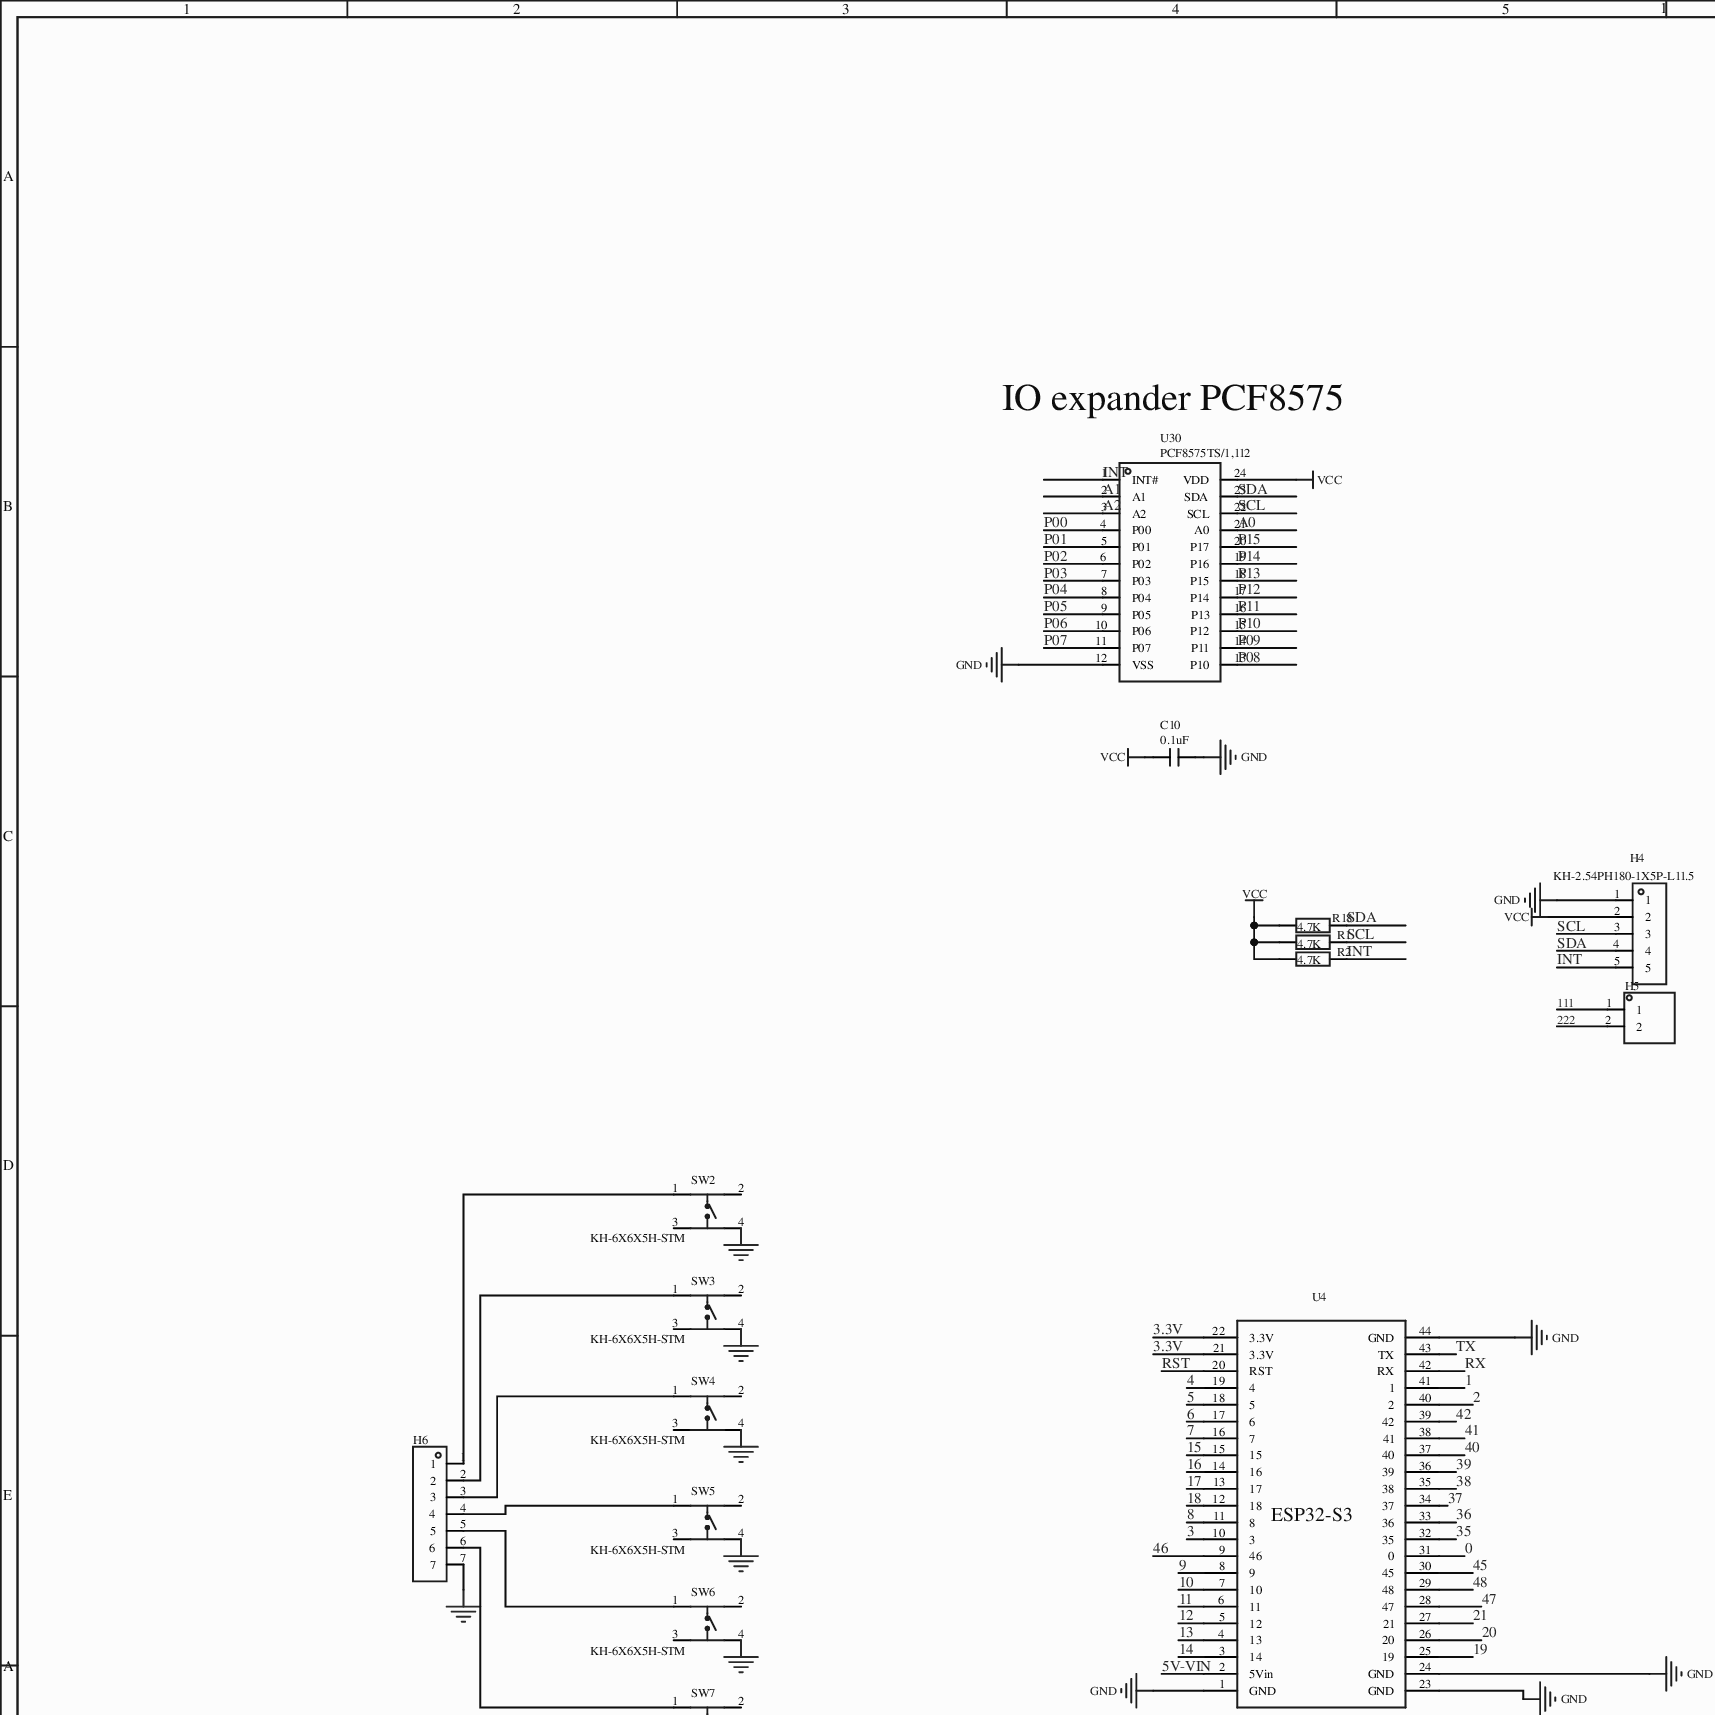
[diagram p0: MISC49879-3.schdoc, top left]
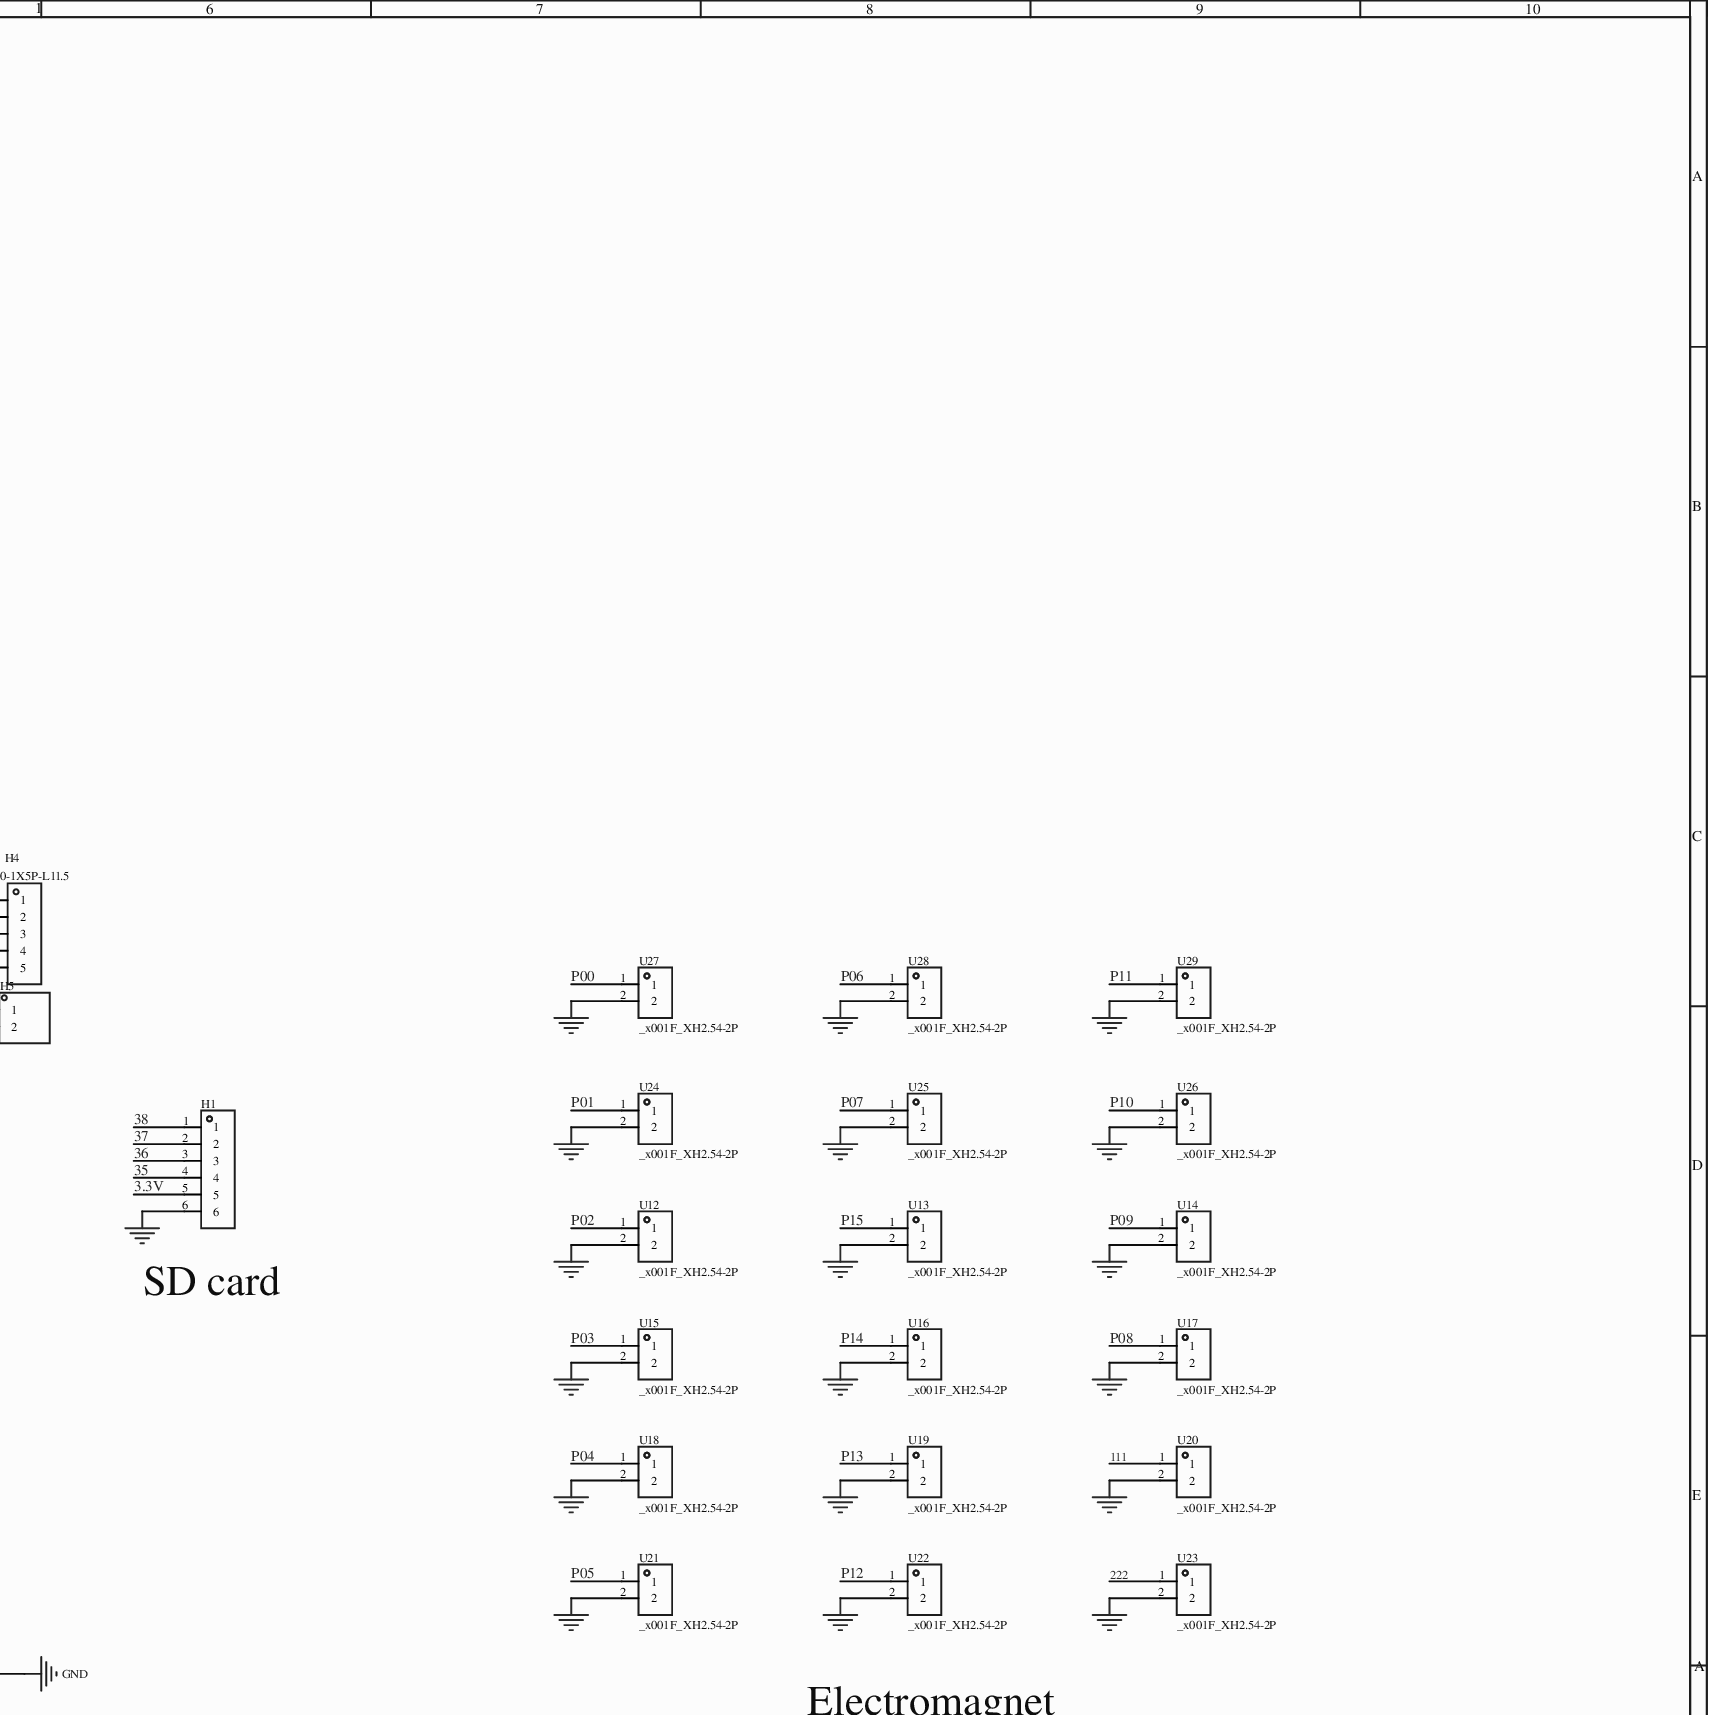
[diagram p1: MISC49879-3.schdoc, top right]
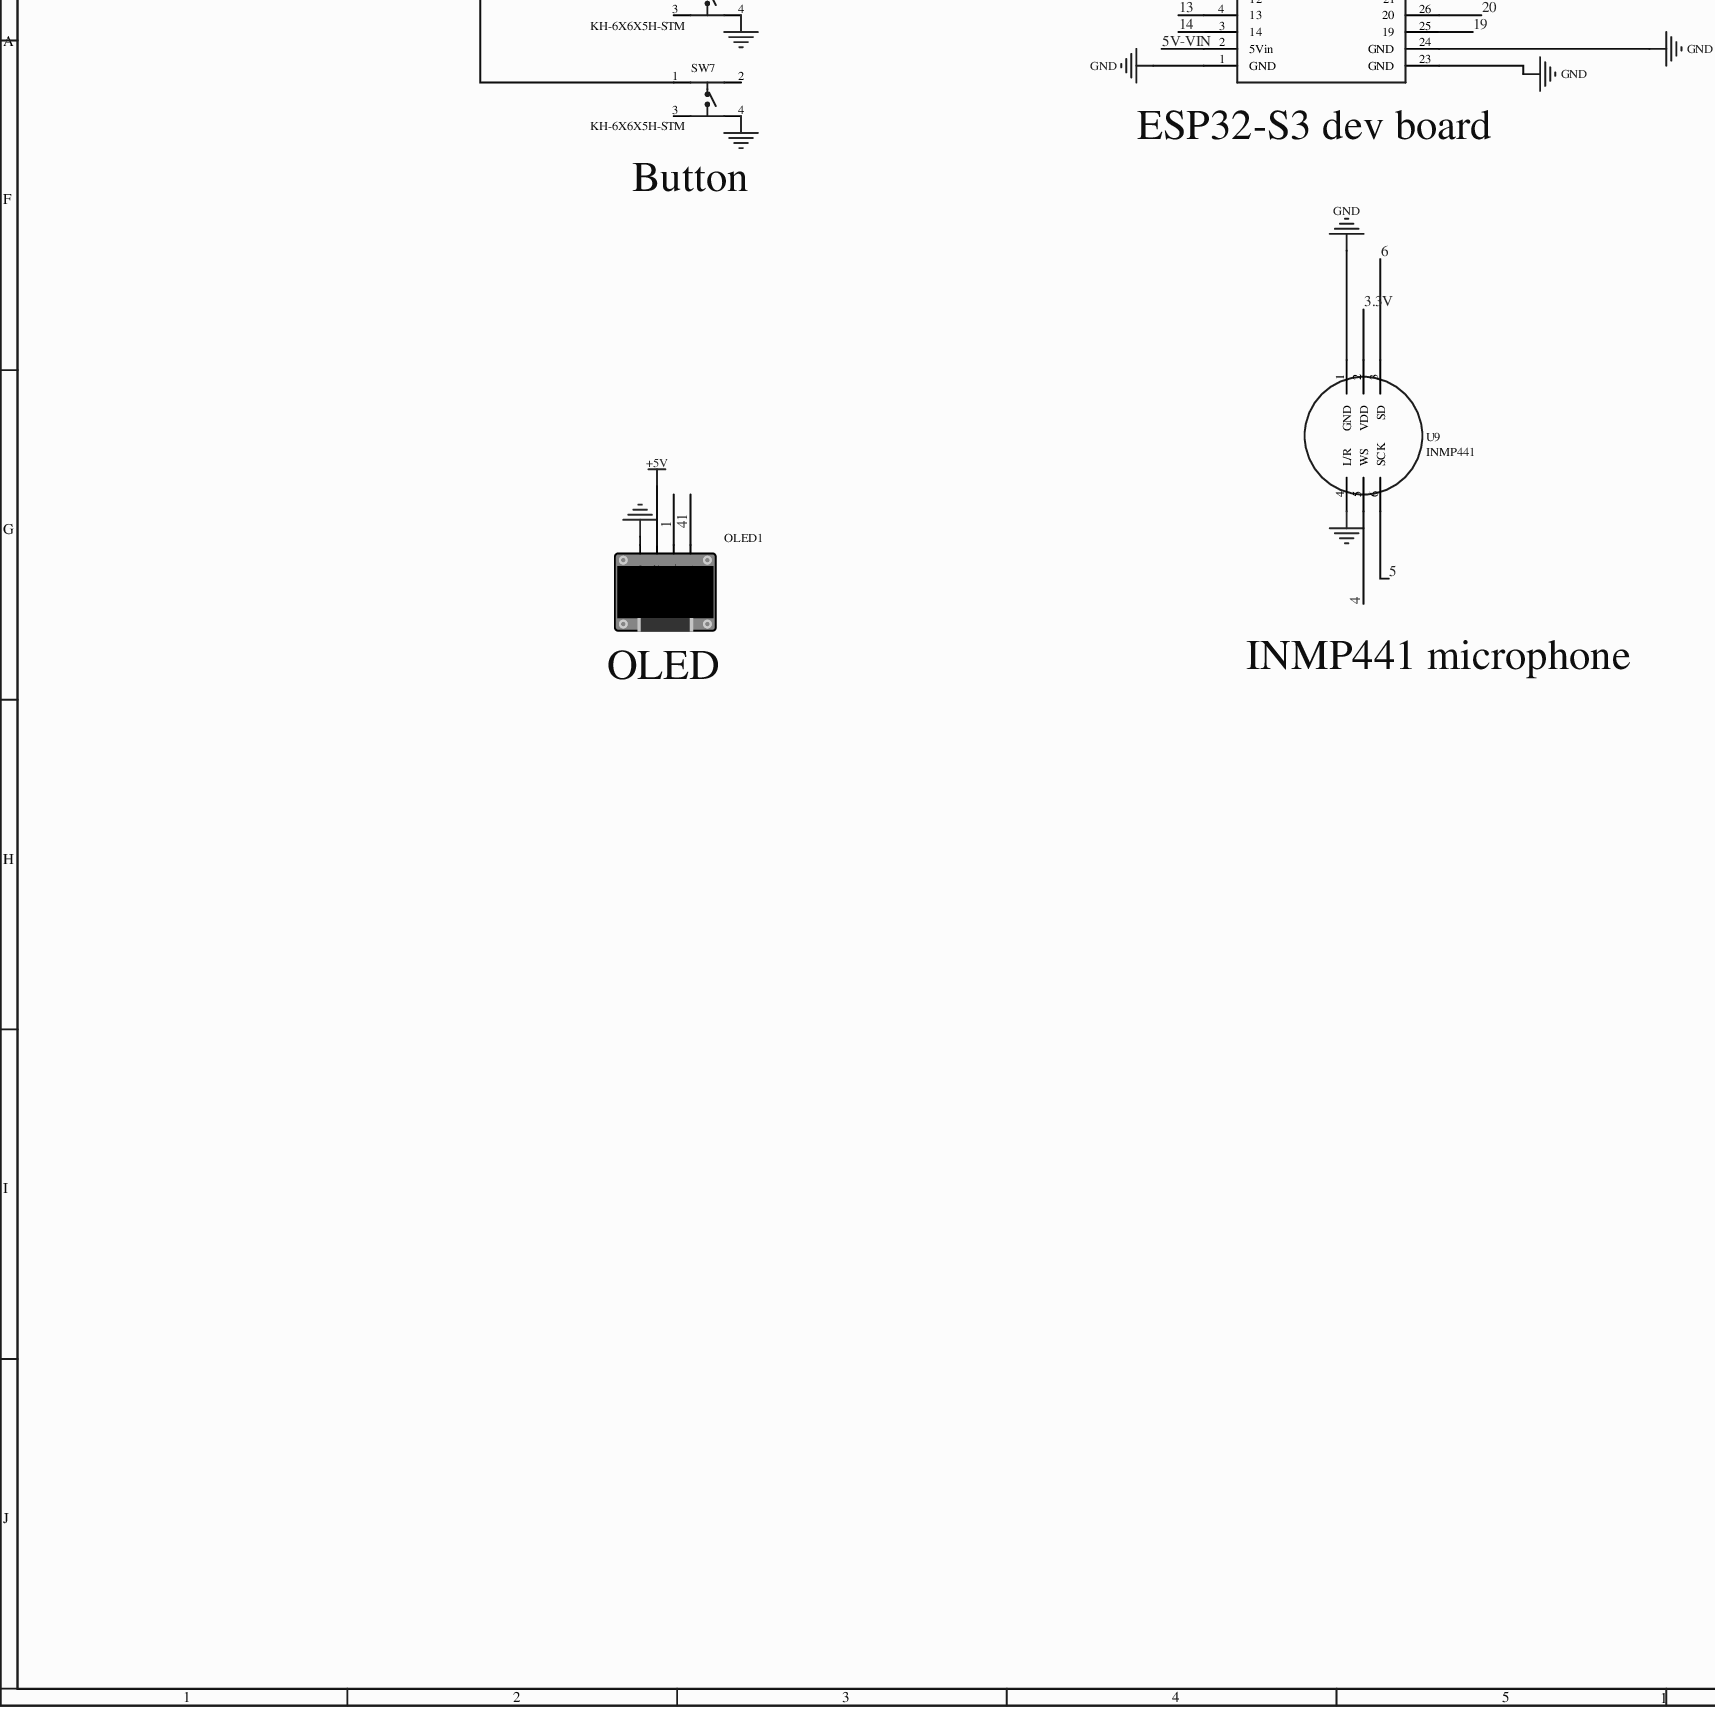
[diagram p2: MISC49879-3.schdoc, bottom left]
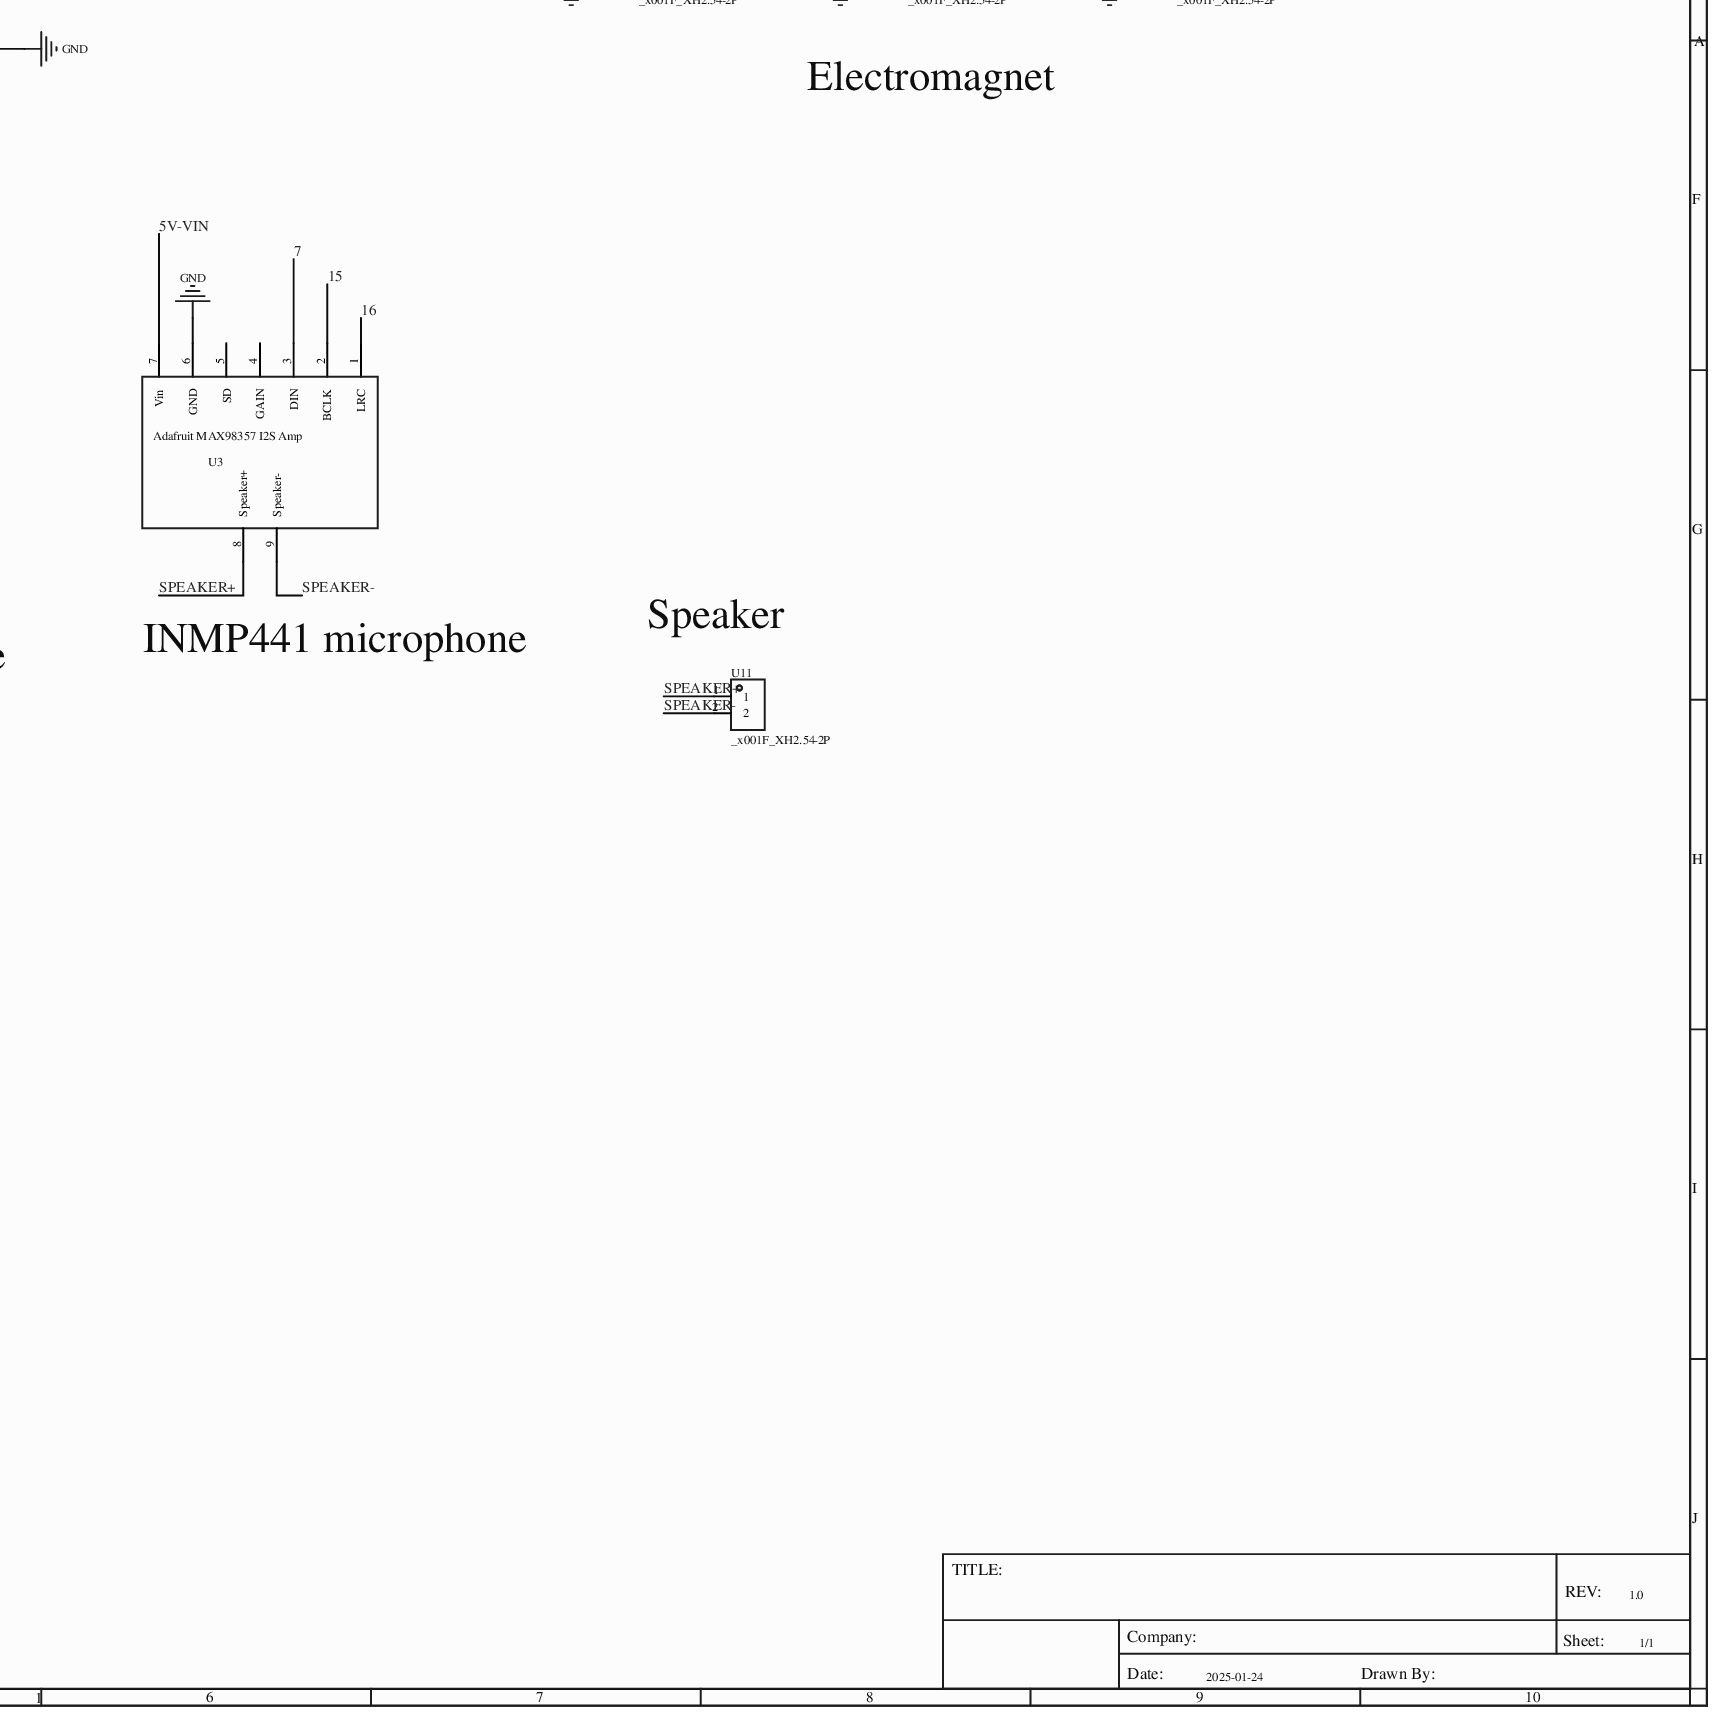
[diagram p3: MISC49879-3.schdoc, bottom right]
# Altium project MISC49879-2.PrjPcb
1 sheet, 38 parts. Net scope: global (net labels, ports and power ports of the same name join across sheets).
Board file: MISC49879.pcbdoc

## Sheet MISC49879-3.schdoc
size 503 x 503 mm; Name: MISC49879; @Project Name: MISC49879; REV: 1.0; Date: 2025-01-24; Sheet: 1/1; @Page No: 1; @Page Count: 1; @Schematic Name: MISC49879; @Board Name: MISC49879; @Update Date: 2025-04-09; @Create Time: 08:27:13; @Update Time: 13:55:30; @Create Date: 2025-04-09

### Parts
C10  0.1uF  [C0603-1]
H1  (no value)  [HDR-TH_6P-P2.54-V-F]
H4  KH-2.54PH180-1X5P-L11.5  [HDR-TH_5P-P2.54-V-M]
H5  (no value)  [HDR-TH_2P-P2.54-V-M-1]
H6  (no value)  [HDR-TH_7P-P2.54-V-M]
OLED1  (no value)  [0.96OLED_4P]
R1  4.7K  [R0603-1]
R2  4.7K  [R0603-1]
R18  4.7K  [R0603-1]
SW2  KH-6X6X5H-STM  [SW-SMD_4P-L6.0-W6.0-P4.50-LS9.0-2]
SW3  KH-6X6X5H-STM  [SW-SMD_4P-L6.0-W6.0-P4.50-LS9.0-2]
SW4  KH-6X6X5H-STM  [SW-SMD_4P-L6.0-W6.0-P4.50-LS9.0-2]
SW5  KH-6X6X5H-STM  [SW-SMD_4P-L6.0-W6.0-P4.50-LS9.0-2]
SW6  KH-6X6X5H-STM  [SW-SMD_4P-L6.0-W6.0-P4.50-LS9.0-2]
SW7  KH-6X6X5H-STM  [SW-SMD_4P-L6.0-W6.0-P4.50-LS9.0-2]
U3  Adafruit MAX98357 I2S Amp  [MAX98357 I2S AMP MODULE]
U4  NO  [ESP32S3]  (value not drawn)
U9  INMP441  [INMP441]
U11  _x001F_XH2.54-2P  [CONN-TH_2P-P2.54-V]
U12  _x001F_XH2.54-2P  [CONN-TH_2P-P2.54-V]
U13  _x001F_XH2.54-2P  [CONN-TH_2P-P2.54-V]
U14  _x001F_XH2.54-2P  [CONN-TH_2P-P2.54-V]
U15  _x001F_XH2.54-2P  [CONN-TH_2P-P2.54-V]
U16  _x001F_XH2.54-2P  [CONN-TH_2P-P2.54-V]
U17  _x001F_XH2.54-2P  [CONN-TH_2P-P2.54-V]
U18  _x001F_XH2.54-2P  [CONN-TH_2P-P2.54-V]
U19  _x001F_XH2.54-2P  [CONN-TH_2P-P2.54-V]
U20  _x001F_XH2.54-2P  [CONN-TH_2P-P2.54-V]
U21  _x001F_XH2.54-2P  [CONN-TH_2P-P2.54-V]
U22  _x001F_XH2.54-2P  [CONN-TH_2P-P2.54-V]
U23  _x001F_XH2.54-2P  [CONN-TH_2P-P2.54-V]
U24  _x001F_XH2.54-2P  [CONN-TH_2P-P2.54-V]
U25  _x001F_XH2.54-2P  [CONN-TH_2P-P2.54-V]
U26  _x001F_XH2.54-2P  [CONN-TH_2P-P2.54-V]
U27  _x001F_XH2.54-2P  [CONN-TH_2P-P2.54-V]
U28  _x001F_XH2.54-2P  [CONN-TH_2P-P2.54-V]
U29  _x001F_XH2.54-2P  [CONN-TH_2P-P2.54-V]
U30  PCF8575TS/1,112  [SSOP-24_L8.2-W5.3-P0.65-LS7.8-BL]

### Nets
+5V: OLED1.2(VCC)
GND: C10.1 H1.6 H4.1 H6.7 OLED1.1(GND) SW2.4 SW3.4 SW4.4 SW5.4 SW6.4 SW7.4 U3.6(GND) U4.1(GND) U4.23(GND) U4.24(GND) U4.44(GND) U9.1(GND) U9.4(L/R) U12.2 U13.2 U14.2 U15.2 U16.2 U17.2 U18.2 U19.2 U20.2 U21.2 U22.2 U23.2 U24.2 U25.2 U26.2 U27.2 U28.2 U29.2 U30.12(VSS)
VCC: C10.2 H4.2 R1.2 R2.2 R18.2 U30.24(VDD)
0: U4.31(0)
1: OLED1.3(SCL) U4.41(1)
2: U4.40(2)
3: U4.10(3)
3.3V: H1.5 U4.21(3.3V) U4.22(3.3V) U9.2(VDD)
4: U4.19(4) U9.5(WS)
5: U4.18(5) U9.6(SCK)
5V-VIN: U3.7(Vin) U4.2(5Vin)
6: U4.17(6) U9.3(SD)
7: U3.3(DIN) U4.16(7)
8: U4.11(8)
9: U4.8(9)
10: U4.7(10)
11: U4.6(11)
12: U4.5(12)
13: U4.4(13)
14: U4.3(14)
15: U3.2(BCLK) U4.15
16: U3.1(LRC) U4.14(16)
17: U4.13(17)
18: U4.12(18)
19: U4.25(19)
20: U4.26(20)
21: U4.27(21)
35: H1.4 U4.32(35)
36: H1.3 U4.33(36)
37: H1.2 U4.34(37)
38: H1.1 U4.35(38)
39: U4.36(39)
40: U4.37(40)
41: OLED1.4(SDA) U4.38(41)
42: U4.39(42)
45: U4.30(45)
46: U4.9(46)
47: U4.28(47)
48: U4.29(48)
111: H5.1 U20.1
222: H5.2 U23.1
A0: U30.21(A0)
A1: U30.2(A1)
A2: U30.3(A2)
INT: H4.5 R2.1 U30.1(INT#)
P00: U27.1 U30.4(P00)
P01: U24.1 U30.5(P01)
P02: U12.1 U30.6(P02)
P03: U15.1 U30.7(P03)
P04: U18.1 U30.8(P04)
P05: U21.1 U30.9(P05)
P06: U28.1 U30.10(P06)
P07: U25.1 U30.11(P07)
P08: U17.1 U30.13(P10)
P09: U14.1 U30.14(P11)
P10: U26.1 U30.15(P12)
P11: U29.1 U30.16(P13)
P12: U22.1 U30.17(P14)
P13: U19.1 U30.18(P15)
P14: U16.1 U30.19(P16)
P15: U13.1 U30.20(P17)
RST: U4.20(RST)
RX: U4.42(RX)
SCL: H4.3 R1.1 U30.22(SCL)
SDA: H4.4 R18.1 U30.23(SDA)
SPEAKER+: U3.8(Speaker+) U11.1
SPEAKER-: U3.9(Speaker-) U11.2
TX: U4.43(TX)
NetH6_1: H6.1 SW2.1
NetH6_2: H6.2 SW3.1
NetH6_3: H6.3 SW4.1
NetH6_4: H6.4 SW5.1
NetH6_5: H6.5 SW6.1
NetH6_6: H6.6 SW7.1

Not connected (* = marked no-connect by the designer): SW2 2 3; SW3 2 3; SW4 2 3; SW5 2 3; SW6 2 3; SW7 2 3; U3 4(GAIN) 5(SD)

### Notes on the sheet
- (near U30) IO expander PCF8575
- (near H1) SD card
- (near U4) ESP32-S3 dev board
- Electromagnet
- (near SW7) Button
- (near U11) Speaker
- OLED
- INMP441 microphone
- 1
- 2
- 3
- 4
- 5
- 6
- 7
- 8
- 9
- 10
- A
- B
- C
- D
- E
- F
- G
- H
- I
- J
- TITLE:
- Company:
- Sheet:
- REV:
- 1.0
- 1/1
- Date:
- 2025-01-24
- Drawn By:

### Library data of the parts
C10 = 0.1uF: Convert to PCB: yes; Origin Footprint: C0603-1; Device: 0.1uF; Symbol: 0.1uF; Add into BOM: yes; FootprintName: C0603-1
H1 = HDR-F_2.54_1x6P: Symbol: Header-Female-2.54_1x6; ConvertToPcb: yes; ModelId: 0f5bcf94dcda47d085f24cdca1696fe9; ModelTransform: 619.684,94.488,0,0,0,0,0,0,-125.984; Device: HDR-F_2.54_1x6P; AddInBom: yes; SupplierPart: C40877; Supplier Footprint: 插件; FootprintName: HDR-TH_6P-P2.54-V-F; ModelName: HDR-TH_6P-P2.54-V-F
H4 = KH-2.54PH180-1X5P-L11.5: Manufacturer: kinghelm(金航标); Convert to PCB: yes; Origin Footprint: HDR-TH_5P-P2.54-V-M; Device: KH-2.54PH180-1X5P-L11.5; Symbol: KH-2.54PH180-1X5P-L11.5; Add into BOM: yes; Supplier: LCSC; SupplierPart: C2932699; ManufacturerPart: KH-2.54PH180-1X5P-L11.5; FootprintName: HDR-TH_5P-P2.54-V-M
H5 = HDR-M_2.54_1x2P: Symbol: 210S-1*2P L=11.6MMGold-plated black; ConvertToPcb: yes; ModelId: 79b2e9f2d70a4d68a1b7098f27c6d4c5; ModelName: HDR-M-2.54_1x2; ModelTransform: 200,100,0,0,0,0,0,0,-118.11; Device: HDR-M_2.54_1x2P; AddInBom: yes; SupplierPart: C124375; Supplier Footprint: 插件; FootprintName: HDR-TH_2P-P2.54-V-M-1
H6 = HDR-M_2.54_1x7P: Symbol: PZ254V-11-07P; ConvertToPcb: yes; ModelId: 3f496cdc752348c6a5e9157bbaceaf96; ModelName: HDR-TH_7P-P2.54-M-LI-1X7P; ModelTransform: 690.1561,98.425,0,0,0,0,0,0,-118.11; Device: HDR-M_2.54_1x7P; AddInBom: yes; SupplierPart: C492406; Supplier Footprint: 插件; FootprintName: HDR-TH_7P-P2.54-V-M
OLED1 = 0.96OLED模块_4P: Device: 0.96OLED module_4P; ConvertToPcb: yes; ModelId: 79c000fdb68d45a296c2e9bedf4f9055; ModelTransform: 1393.69792,1318.895,0,0,0,0,0,-560.079,-137.795; AddInBom: yes; SymbolName: 0.96OLED module_4P; FootprintName: 0.96OLED_4P; Supplier Footprint: 插件; ModelName: 0.96OLED_4P
R1 R2 R18 = 4.7K: Convert to PCB: yes; Origin Footprint: R0603-1; Device: 4.7K; Symbol: 4.7K; Add into BOM: yes; FootprintName: R0603-1
SW2-SW7 = KH-6X6X5H-STM: Structure: SPST; Actuator: round button; Mounting: upright SMD; Length: 6mm; Width: 6mm; Height: 5mm; With bracket: no; Contact current: 50mA; Rated voltage (DC): 12V; Mechanical life: 8 ten-thousand cycles;; Manufacturer: kinghelm(金航标); AddInBom: yes; ModelId: fbf4ceca6c4742d48614ab6a891ef981; ModelName: SW-SMD_4P-L6.0-W6.0-P4.50-LS11.0; ModelTransform: 330.708,251.968,0,0,0,0,0,-0.005,0; Actuator/Cap Color: Black; Pin Style: Gull-wing; Symbol: KH-6X6X5H-STM; Device: KH-6X6X5H-STM; LCSC Part Name: 6*6*5mm 立贴 轻触开关; SupplierPart: C2837531; ManufacturerPart: KH-6X6X5H-STM; Supplier Footprint: SMD; JLCPCB Part Class: Extended library; Datasheet: https://atta.szlcsc.com/upload/public/pdf/source/20210608/C2837531_45E87AB996CE723B09405FF2EA209C4C.pdf; Supplier: LCSC; ConvertToPcb: yes; FootprintName: SW-SMD_4P-L6.0-W6.0-P4.50-LS9.0-2; Circuit: SPST; Actuator Style: Round button; Mounting Style: Upright SMD; Switch Length: 6mm; Switch Width: 6mm; Switch Height: 5mm; Strike Gundam: No; Contact Current: 50mA; Voltage Rating (DC): 12V; Mechanical Life: 8 ten-thousand cycles
U3 = Adafruit MAX98357 I2S Amp: Convert to PCB: yes; Origin Footprint: MAX98357 I2S AMP MODULE; Device: Adafruit MAX98357 I2S Amp; Symbol: Adafruit MAX98357 I2S Amp; Manufacturer Part: Adafruit MAX98357 I2S Amp; Add into BOM: yes; FootprintName: MAX98357 I2S AMP MODULE
U4 = NO: Convert to PCB: yes; Origin Footprint: ESP32S3; Device: NO; Symbol: NO; Add into BOM: yes; FootprintName: ESP32S3
U9 = INMP441: Convert to PCB: yes; Origin Footprint: INMP441; Device: INMP441; Symbol: INMP441; Add into BOM: yes; FootprintName: INMP441
U11-U29 = _x001F_XH2.54-2P: AddInBom: yes; ModelId: 4b619f877c224111ac90f050b36c3583; ModelTransform: 295.275,224.409,0,180,0,0,0,17.717,-118.11; Symbol: _X001F_XH2.54-2P; Device: _x001F_XH2.54-2P; LCSC Part Name: _x001F_XH2.54-2P; SupplierPart: C9900016027; ManufacturerPart: _x001F_XH2.54-2P; Supplier Footprint: XH2.54-2P直插; JLCPCB Part Class: Extended library; Supplier: LCSC; ConvertToPcb: yes; FootprintName: CONN-TH_2P-P2.54-V; ModelName: CONN-TH_2P-P2.54-V
U30 = PCF8575TS/1,112: Manufacturer: NXP(恩智浦); Convert to PCB: yes; Origin Footprint: SSOP-24_L8.2-W5.3-P0.65-LS7.8-BL; Device: PCF8575TS/1,112; Symbol: PCF8575TS/1,112; Add into BOM: yes; Supplier: LCSC; SupplierPart: C1542504; ManufacturerPart: PCF8575TS/1,112; FootprintName: SSOP-24_L8.2-W5.3-P0.65-LS7.8-BL